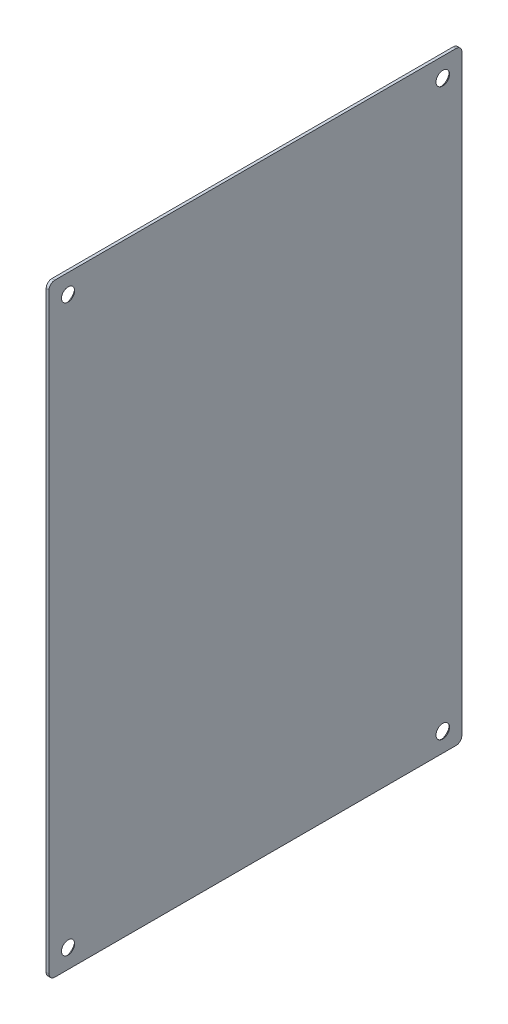
from build123d import *

# Parameters (mm, degrees)
SKETCH_1_W                       = 316.6
SKETCH_1_H                       = 216.5
EXTRUDE_1_DEPTH                  = 1.5
HOLE_WIZARD_1_AT_2_COUNT         = 2
HOLE_WIZARD_1_AT_2_PITCH         = 296.6
HOLE_WIZARD_7_1_7_1_1_AT_2_COUNT = 2
HOLE_WIZARD_7_1_7_1_1_AT_2_PITCH = 296.6
FILLET_1_R                       = 3


with BuildPart() as part:
    # 草图1 → 凸台-拉伸1 (new body)
    with BuildSketch(Plane(origin=(2615.929548806, 0, 0), x_dir=(0, -1, 0), z_dir=(-1, 0, 0))):
        with Locations((-1211, 190.894615796)):
            Rectangle(SKETCH_1_W, SKETCH_1_H)
    extrude(amount=-EXTRUDE_1_DEPTH)

    # 草图2 → 孔1 (revolve, cut)
    with BuildSketch(Plane(origin=(2615.929548806, 1062.7, 289.144615796), x_dir=(0, 0, 1), z_dir=(0, 1, 0))):
        Polygon((0, 0), (0, 1.5), (3.45, 1.5), (4.95, 0), align=None)
    hole_wizard_1 = revolve(axis=Axis((2725.929548806, 1062.7, 289.144615796), (-1, 0, 0)), mode=Mode.SUBTRACT)

    # 孔1 at 2: 孔1 ×2
    with Locations(*[(0, i * HOLE_WIZARD_1_AT_2_PITCH, 0) for i in range(1, HOLE_WIZARD_1_AT_2_COUNT)]):
        add(hole_wizard_1, mode=Mode.SUBTRACT)

    # 草图4 → Ø7.1 (7.1) 直径孔1 (revolve, cut)
    with BuildSketch(Plane(origin=(2615.929548806, 1359.3, 92.644615796), x_dir=(0, 0, 1), z_dir=(0, 1, 0))):
        Polygon((0, 0), (0, 1.5), (3.55, 1.5), (3.55, 1.4), (4.95, 0), align=None)
    hole_wizard_7_1_7_1_1 = revolve(axis=Axis((2609.579548806, 1359.3, 92.644615796), (1, 0, 0)), mode=Mode.SUBTRACT)

    # Ø7.1 (7.1) 直径孔1 at 2: Ø7.1 (7.1) 直径孔1 ×2
    with Locations(*[(0, -i * HOLE_WIZARD_7_1_7_1_1_AT_2_PITCH, 0) for i in range(1, HOLE_WIZARD_7_1_7_1_1_AT_2_COUNT)]):
        add(hole_wizard_7_1_7_1_1, mode=Mode.SUBTRACT)

    # 圆角1
    fillet_1_edges = [part.edges().sort_by_distance(p)[0] for p in [
        (2616.679548806, 1052.7, 299.144615796),
        (2616.679548806, 1052.7, 82.644615796),
        (2616.679548806, 1369.3, 82.644615796),
        (2616.679548806, 1369.3, 299.144615796),
    ]]
    fillet(fillet_1_edges, radius=FILLET_1_R)


solid = part.part
